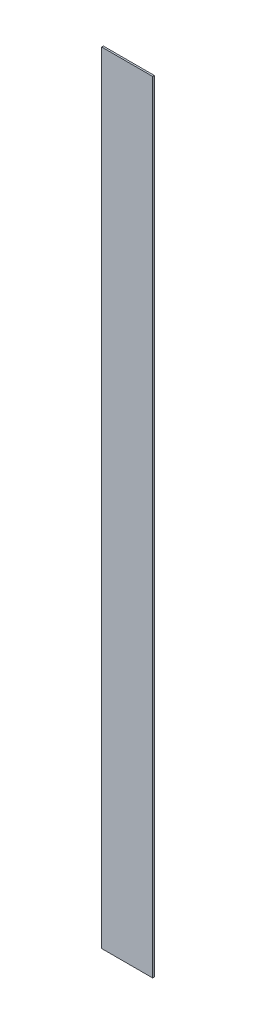
from build123d import *

# Parameters (mm, degrees)
SKETCH_1_W      = 151
SKETCH_1_H      = 2310
EXTRUDE_1_DEPTH = 5


with BuildPart() as part:
    # 草图1 → 凸台-拉伸1 (new body)
    with BuildSketch(Plane.XY):
        Rectangle(SKETCH_1_W, SKETCH_1_H)
    extrude(amount=EXTRUDE_1_DEPTH)


solid = part.part
